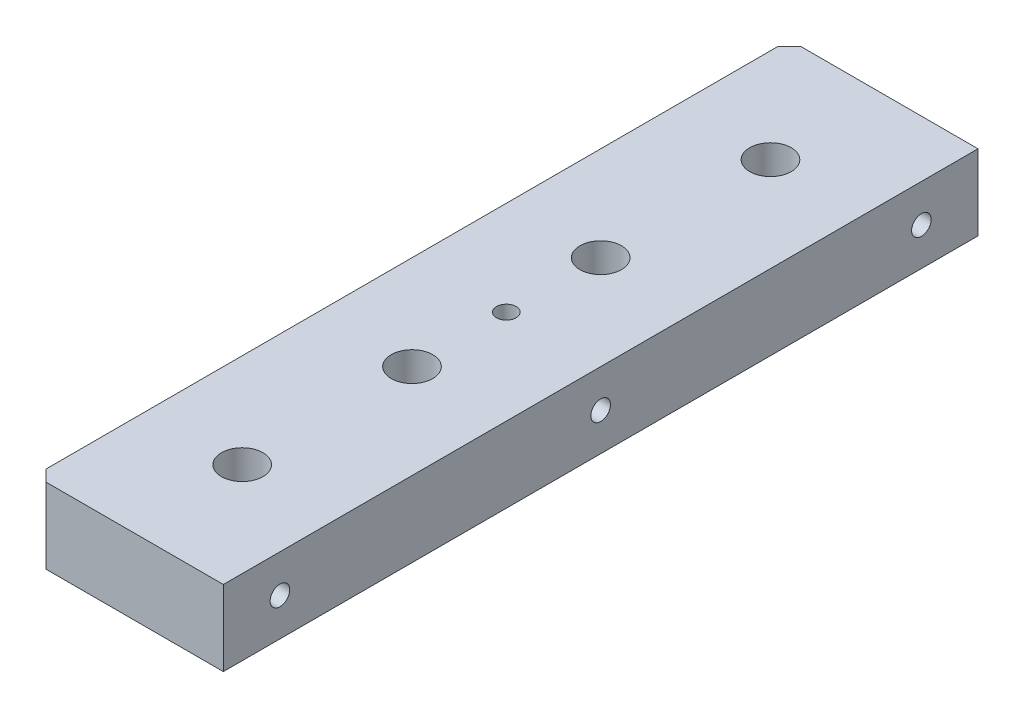
SolidWorks part; units mm, degrees
material "6061"
ref_plane "前视基准面" through (0, 0, 0) normal (0, 0, 1) x (1, 0, 0)
ref_plane "上视基准面" through (0, 0, 0) normal (0, 1, 0) x (1, 0, 0)
ref_plane "右视基准面" through (0, 0, 0) normal (1, 0, 0) x (0, 0, -1)
sketch "草图1" plane through (0, 0, 0) normal (0, 1, 0) x (1, 0, 0)
  line L1 (25, -100) -> (-25, -100)
  line L2 (25, -100) -> (25, 100)
  line L3 (25, 100) -> (-25, 100)
  line L4 (-25, -100) -> (-25, 100)
  line L5 (25, -100) -> (-25, 100) construction
  line L6 (25, 100) -> (-25, -100) construction
  point P0 (0, 0)
  dimension "D1" = 50
  dimension "D2" = 200
extrude "凸台-拉伸1" add sketch "草图1" along normal mid plane 20
hole_wizard "M6 六角凹头螺钉的柱形沉头孔1" positions "草图2" profile "草图3" counterbore size "M6" standard "ISO" end condition through all
sketch "草图2" plane through (0, 10, 0) normal (0, 1, 0) x (1, 0, 0)
  line L0 (0, 100) -> (0, -100) construction
  line L1 (25, 100) -> (-25, 100) construction
  line L2 (-25, -100) -> (25, -100) construction
  line L4 (25, 0) -> (-58.9398, 0) construction
  line L5 (25, -100) -> (25, 100) construction
  point P0 (0, 70)
  point P2 (0, -70)
  point P21 (0, 25)
  point P23 (0, -25)
  dimension "D1" = 140
  dimension "D2" = 50
sketch "草图3" plane through (0, 10, -70) normal (1, 0, 0) x (0, 0, 1)
  line L0 (0, 0) -> (0, 20)
  line L1 (0, 20) -> (3.3, 20)
  line L3 (3.3, 20) -> (3.3, 8)
  line L4 (3.3, 8) -> (5.5, 8)
  line L5 (5.5, 8) -> (5.5, 0)
  line L7 (5.5, 0) -> (0, 0)
  line L11 (0, -6.35) -> (0, 107.95) construction
  dimension "通孔孔直径" = 6.6
  dimension "通孔孔深度" = 20
  dimension "柱形沉头孔直径" = 11
  dimension "柱形沉头孔深度" = 8
hole_wizard "M6 螺纹孔1" positions "草图4" profile "草图5" tap size "M6" standard "ISO"
sketch "草图4" plane through (25, 0, 0) normal (1, 0, 0) x (0, 0, -1)
  point P0 (-85, 0)
  point P3 (0, 0)
  point P6 (85, 0)
cosmetic thread "孔螺蚊线1" parameters "D1"=12, "D2"=6
cosmetic thread "孔螺蚊线2" parameters "D1"=12, "D2"=6
cosmetic thread "孔螺蚊线3" parameters "D1"=12, "D2"=6
sketch "草图5" plane through (25, 0, 85) normal (0, 1, 0) x (0, 0, -1)
  line L0 (0, 0) -> (0, 16.5622)
  line L1 (0, 16.5622) -> (2.6, 15)
  line L2 (2.6, 15) -> (2.6, 0)
  line L5 (2.6, 0) -> (0, 0)
  line L10 (0, 16.5622) -> (-2.6, 15) construction
  line L11 (0, -6.35) -> (0, 107.95) construction
  dimension "螺纹孔钻头直径" = 5.2
  dimension "螺纹孔钻头深度" = 15
  dimension "导头角度" = 118
hole_wizard "M6 六角凹头螺钉的柱形沉头孔2" positions "草图6" profile "草图7" counterbore size "M6" standard "ISO" end condition through all
sketch "草图6" plane through (0, -10, 0) normal (0, -1, 0) x (-1, 0, 0)
  point P0 (0, 0)
sketch "草图7" plane through (0, -10, 0) normal (1, 0, 0) x (0, 0, -1)
  line L0 (0, 0) -> (0, 20)
  line L1 (0, 20) -> (2.6, 20)
  line L3 (2.6, 20) -> (2.6, 6.4)
  line L4 (2.6, 6.4) -> (5.5, 6.4)
  line L5 (5.5, 6.4) -> (5.5, 0)
  line L7 (5.5, 0) -> (0, 0)
  line L11 (0, -6.35) -> (0, 107.95) construction
  dimension "通孔孔直径" = 5.2
  dimension "通孔孔深度" = 20
  dimension "柱形沉头孔直径" = 11
  dimension "柱形沉头孔深度" = 6.4
chamfer "倒角1" distance 3 angle 45 2 edges at (-25, 0, 100) (-25, 0, -100)
